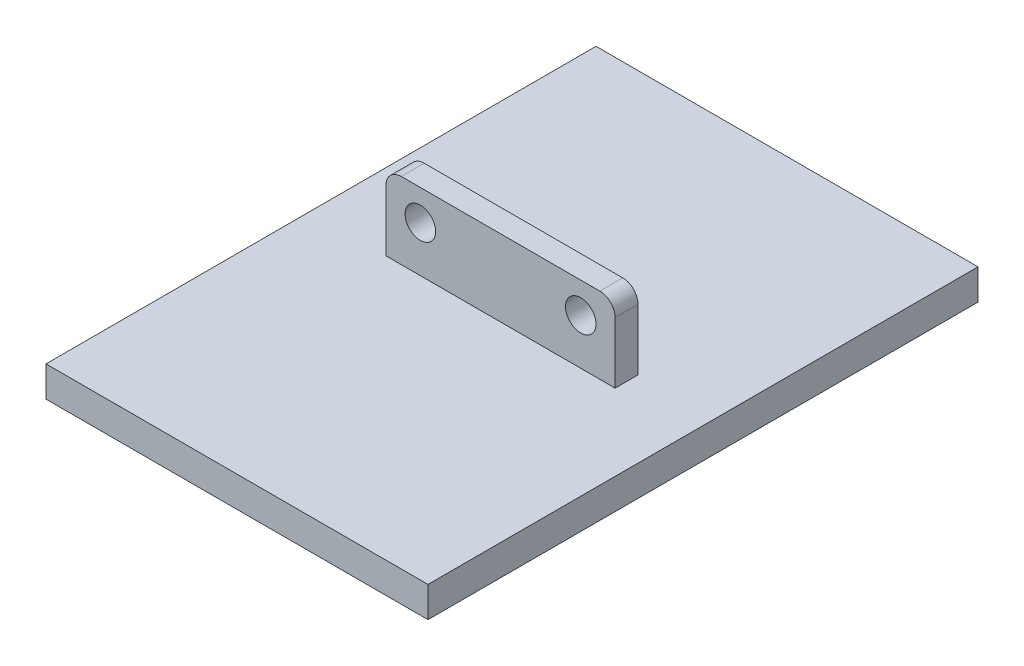
from build123d import *

# Parameters (mm, degrees)
SKETCH1_W           = 250
SKETCH1_H           = 360
BOSS_EXTRUDE1_DEPTH = 20
SKETCH2_W           = 150
SKETCH2_H           = 15
BOSS_EXTRUDE2_DEPTH = 50
FILLET1_R           = 10
SKETCH3_R           = 10
CUT_EXTRUDE1_DEPTH  = 236.968747931


with BuildPart() as part:
    # Sketch1 → Boss-Extrude1 (new body)
    with BuildSketch(Plane(origin=(0, 0, 0), x_dir=(1, 0, 0), z_dir=(0, 1, 0))):
        Rectangle(SKETCH1_W, SKETCH1_H)
    extrude(amount=BOSS_EXTRUDE1_DEPTH)

    # Sketch2 → Boss-Extrude2 (add)
    with BuildSketch(Plane(origin=(0, 20, 0), x_dir=(1, 0, 0), z_dir=(0, 1, 0))):
        Rectangle(SKETCH2_W, SKETCH2_H)
    extrude(amount=BOSS_EXTRUDE2_DEPTH)

    # Fillet1
    fillet1_edges = [part.edges().sort_by_distance(p)[0] for p in [
        (-75, 70, 0),
        (75, 70, 0),
    ]]
    fillet(fillet1_edges, radius=FILLET1_R)

    # Sketch3 → Cut-Extrude1 (cut, through all)
    with BuildSketch(Plane.XY.offset(7.5)):
        with Locations((52.5, 50)):
            Circle(SKETCH3_R)
        with Locations((-52.5, 50)):
            Circle(SKETCH3_R)
    extrude(amount=-CUT_EXTRUDE1_DEPTH, mode=Mode.SUBTRACT)


solid = part.part
